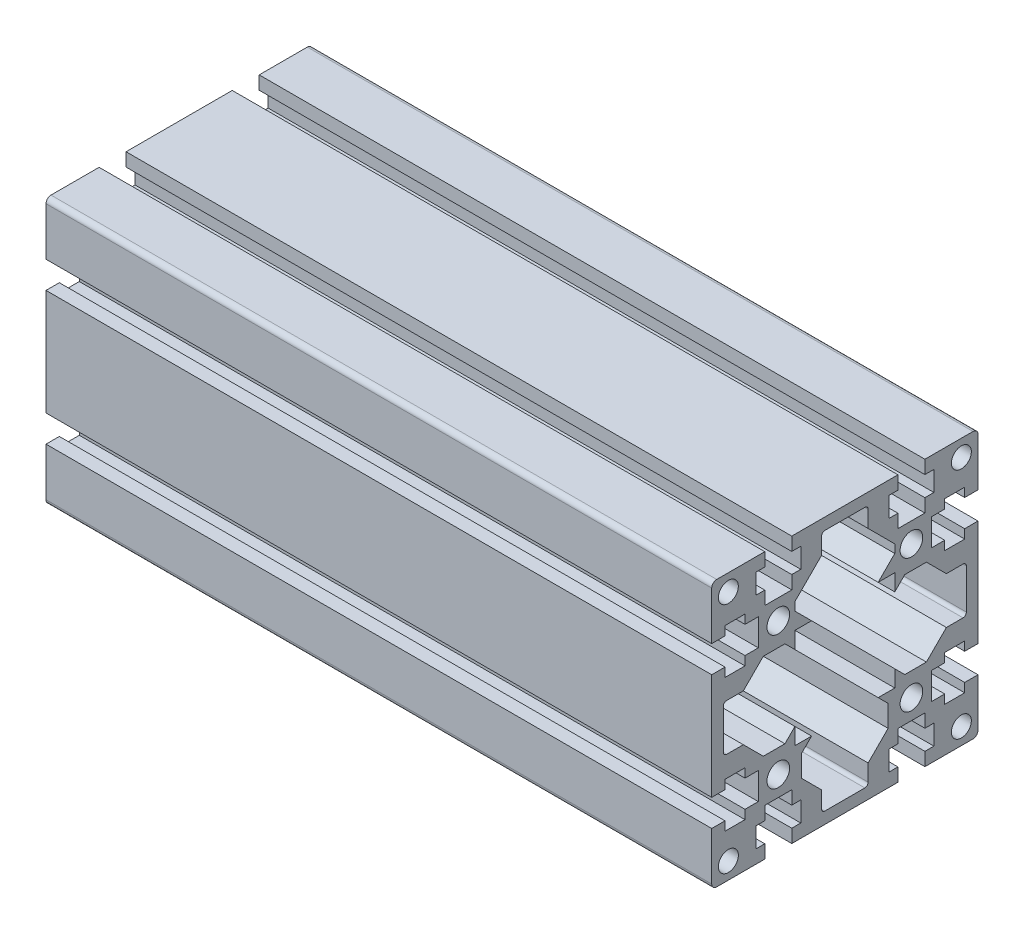
from build123d import *

# Parameters (mm, degrees)
SKETCH1_R                                 = 3.4
SKETCH1_R_2                               = 3
ALUMINIUM_PROFILE_80_X_80G_X_R1_5_1_DEPTH = 200
SKETCH10_R                                = 3
CUT_EXTRUDE1_DEPTH                        = 208.846096908


with BuildPart() as part:
    # Sketch1 → Aluminium profile 80 X 80G X R1.5(1) (new body)
    with BuildSketch(Plane.YZ.offset(-530.344827586)):
        with BuildLine():
            Line((-24.05, 40), (-24.05, 36))
            Line((-24.05, 36), (-26.75, 36))
            Line((-26.75, 36), (-26.75, 30))
            Line((-26.75, 30), (-24.05, 30))
            Line((-24.05, 30), (-24.05, 26))
            Line((-24.05, 26), (-15.95, 26))
            Line((-15.95, 26), (-15.95, 30))
            Line((-15.95, 30), (-13.25, 30))
            Line((-13.25, 30), (-13.25, 36))
            Line((-13.25, 36), (-15.95, 36))
            Line((-15.95, 36), (-15.95, 40))
            Line((-15.95, 40), (15.95, 40))
            Line((15.95, 40), (15.95, 36))
            Line((15.95, 36), (13.25, 36))
            Line((13.25, 36), (13.25, 30))
            Line((13.25, 30), (15.95, 30))
            Line((15.95, 30), (15.95, 26))
            Line((15.95, 26), (24.05, 26))
            Line((24.05, 26), (24.05, 30))
            Line((24.05, 30), (26.75, 30))
            Line((26.75, 30), (26.75, 36))
            Line((26.75, 36), (24.05, 36))
            Line((24.05, 36), (24.05, 40))
            Line((24.05, 40), (38.5, 40))
            ThreePointArc((38.5, 40), (39.560660172, 39.560660172), (40, 38.5))
            Line((40, 38.5), (40, 24.05))
            Line((40, 24.05), (36, 24.05))
            Line((36, 24.05), (36, 26.75))
            Line((36, 26.75), (30, 26.75))
            Line((30, 26.75), (30, 24.05))
            Line((30, 24.05), (26, 24.05))
            Line((26, 24.05), (26, 15.95))
            Line((26, 15.95), (30, 15.95))
            Line((30, 15.95), (30, 13.25))
            Line((30, 13.25), (36, 13.25))
            Line((36, 13.25), (36, 15.95))
            Line((36, 15.95), (40, 15.95))
            Line((40, 15.95), (40, -15.95))
            Line((40, -15.95), (36, -15.95))
            Line((36, -15.95), (36, -13.25))
            Line((36, -13.25), (30, -13.25))
            Line((30, -13.25), (30, -15.95))
            Line((30, -15.95), (26, -15.95))
            Line((26, -15.95), (26, -24.05))
            Line((26, -24.05), (30, -24.05))
            Line((30, -24.05), (30, -26.75))
            Line((30, -26.75), (36, -26.75))
            Line((36, -26.75), (36, -24.05))
            Line((36, -24.05), (40, -24.05))
            Line((40, -24.05), (40, -38.5))
            ThreePointArc((40, -38.5), (39.560660172, -39.560660172), (38.5, -40))
            Line((38.5, -40), (24.05, -40))
            Line((24.05, -40), (24.05, -36))
            Line((24.05, -36), (26.75, -36))
            Line((26.75, -36), (26.75, -30))
            Line((26.75, -30), (24.05, -30))
            Line((24.05, -30), (24.05, -26))
            Line((24.05, -26), (15.95, -26))
            Line((15.95, -26), (15.95, -30))
            Line((15.95, -30), (13.25, -30))
            Line((13.25, -30), (13.25, -36))
            Line((13.25, -36), (15.95, -36))
            Line((15.95, -36), (15.95, -40))
            Line((15.95, -40), (-15.95, -40))
            Line((-15.95, -40), (-15.95, -36))
            Line((-15.95, -36), (-13.25, -36))
            Line((-13.25, -36), (-13.25, -30))
            Line((-13.25, -30), (-15.95, -30))
            Line((-15.95, -30), (-15.95, -26))
            Line((-15.95, -26), (-24.05, -26))
            Line((-24.05, -26), (-24.05, -30))
            Line((-24.05, -30), (-26.75, -30))
            Line((-26.75, -30), (-26.75, -36))
            Line((-26.75, -36), (-24.05, -36))
            Line((-24.05, -36), (-24.05, -40))
            Line((-24.05, -40), (-38.5, -40))
            ThreePointArc((-38.5, -40), (-39.560660172, -39.560660172), (-40, -38.5))
            Line((-40, -38.5), (-40, -24.05))
            Line((-40, -24.05), (-36, -24.05))
            Line((-36, -24.05), (-36, -26.75))
            Line((-36, -26.75), (-30, -26.75))
            Line((-30, -26.75), (-30, -24.05))
            Line((-30, -24.05), (-26, -24.05))
            Line((-26, -24.05), (-26, -15.95))
            Line((-26, -15.95), (-30, -15.95))
            Line((-30, -15.95), (-30, -13.25))
            Line((-30, -13.25), (-36, -13.25))
            Line((-36, -13.25), (-36, -15.95))
            Line((-36, -15.95), (-40, -15.95))
            Line((-40, -15.95), (-40, 15.95))
            Line((-40, 15.95), (-36, 15.95))
            Line((-36, 15.95), (-36, 13.25))
            Line((-36, 13.25), (-30, 13.25))
            Line((-30, 13.25), (-30, 15.95))
            Line((-30, 15.95), (-26, 15.95))
            Line((-26, 15.95), (-26, 24.05))
            Line((-26, 24.05), (-30, 24.05))
            Line((-30, 24.05), (-30, 26.75))
            Line((-30, 26.75), (-36, 26.75))
            Line((-36, 26.75), (-36, 24.05))
            Line((-36, 24.05), (-40, 24.05))
            Line((-40, 24.05), (-40, 38.5))
            ThreePointArc((-40, 38.5), (-39.560660172, 39.560660172), (-38.5, 40))
            Line((-38.5, 40), (-24.05, 40))
        make_face()
        with Locations((-20, 20)):
            Circle(SKETCH1_R, mode=Mode.SUBTRACT)
        with Locations((20, 20)):
            Circle(SKETCH1_R, mode=Mode.SUBTRACT)
        with Locations((20, -20)):
            Circle(SKETCH1_R, mode=Mode.SUBTRACT)
        with Locations((-20, -20)):
            Circle(SKETCH1_R, mode=Mode.SUBTRACT)
        with Locations((-35, 35)):
            Circle(SKETCH1_R_2, mode=Mode.SUBTRACT)
        with Locations((35, 35)):
            Circle(SKETCH1_R_2, mode=Mode.SUBTRACT)
        with Locations((35, -35)):
            Circle(SKETCH1_R_2, mode=Mode.SUBTRACT)
        with BuildLine():
            Line((-13, 18), (-10, 15))
            Line((-10, 15), (-15, 15))
            Line((-15, 15), (-15, 10))
            Line((-15, 10), (-18, 13))
            Line((-18, 13), (-24.5, 13))
            Line((-24.5, 13), (-30.5, 7))
            Line((-30.5, 7), (-35.5, 7))
            ThreePointArc((-35.5, 7), (-36.207106781, 6.707106781), (-36.5, 6))
            Line((-36.5, 6), (-36.5, -6))
            ThreePointArc((-36.5, -6), (-36.207106781, -6.707106781), (-35.5, -7))
            Line((-35.5, -7), (-30.5, -7))
            Line((-30.5, -7), (-24.5, -13))
            Line((-24.5, -13), (-18, -13))
            Line((-18, -13), (-15, -10))
            Line((-15, -10), (-15, -15))
            Line((-15, -15), (-10, -15))
            Line((-10, -15), (-13, -18))
            Line((-13, -18), (-13, -24.5))
            Line((-13, -24.5), (-7, -30.5))
            Line((-7, -30.5), (-7, -35.5))
            ThreePointArc((-7, -35.5), (-6.707106781, -36.207106781), (-6, -36.5))
            Line((-6, -36.5), (6, -36.5))
            ThreePointArc((6, -36.5), (6.707106781, -36.207106781), (7, -35.5))
            Line((7, -35.5), (7, -30.5))
            Line((7, -30.5), (13, -24.5))
            Line((13, -24.5), (13, -18))
            Line((13, -18), (10, -15))
            Line((10, -15), (15, -15))
            Line((15, -15), (15, -10))
            Line((15, -10), (20, -15))
            Line((20, -15), (22.5, -15))
            Line((22.5, -15), (30.5, -7))
            Line((30.5, -7), (35.5, -7))
            ThreePointArc((35.5, -7), (36.207106781, -6.707106781), (36.5, -6))
            Line((36.5, -6), (36.5, 6))
            ThreePointArc((36.5, 6), (36.207106781, 6.707106781), (35.5, 7))
            Line((35.5, 7), (30.5, 7))
            Line((30.5, 7), (22.5, 15))
            Line((22.5, 15), (20, 15))
            Line((20, 15), (15, 10))
            Line((15, 10), (15, 15))
            Line((15, 15), (10, 15))
            Line((10, 15), (13, 18))
            Line((13, 18), (13, 24.5))
            Line((13, 24.5), (7, 30.5))
            Line((7, 30.5), (7, 35.5))
            ThreePointArc((7, 35.5), (6.707106781, 36.207106781), (6, 36.5))
            Line((6, 36.5), (-6, 36.5))
            ThreePointArc((-6, 36.5), (-6.707106781, 36.207106781), (-7, 35.5))
            Line((-7, 35.5), (-7, 30.5))
            Line((-7, 30.5), (-13, 24.5))
            Line((-13, 24.5), (-13, 18))
        make_face(mode=Mode.SUBTRACT)
    extrude(amount=ALUMINIUM_PROFILE_80_X_80G_X_R1_5_1_DEPTH)

    # Sketch10 → Cut-Extrude1 (cut, through all)
    with BuildSketch(Plane(origin=(-330.344827586, 0, 0), x_dir=(0, 0, -1), z_dir=(1, 0, 0))):
        with Locations((35, -35)):
            Circle(SKETCH10_R)
    extrude(amount=-CUT_EXTRUDE1_DEPTH, mode=Mode.SUBTRACT)


solid = part.part
